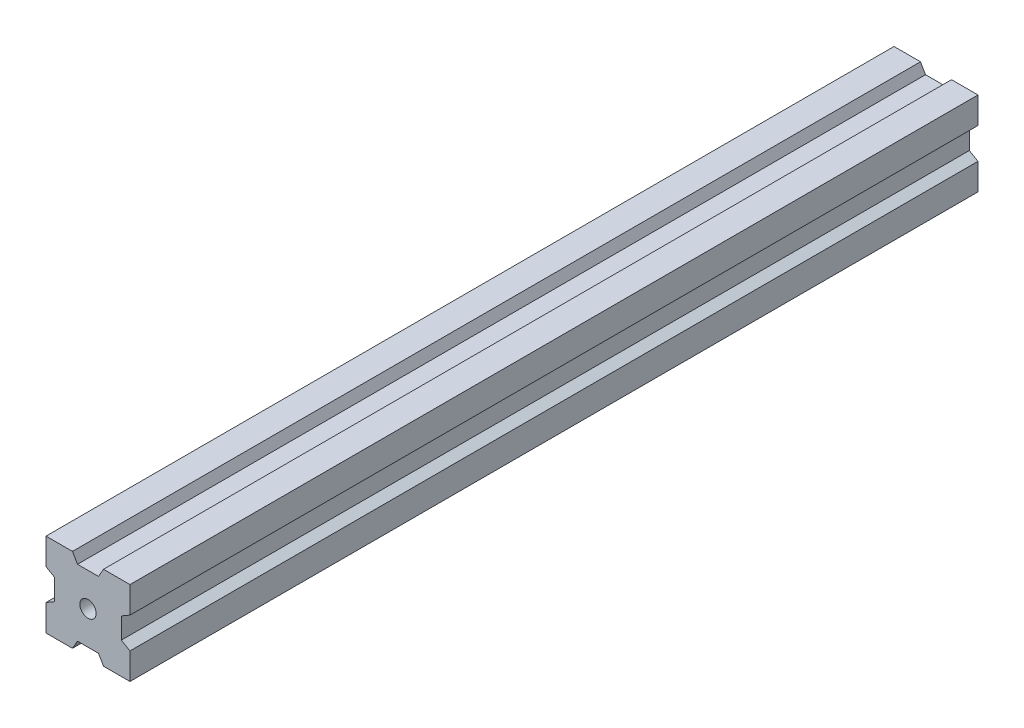
SolidWorks part; units mm, degrees
ref_plane "前视基准面" through (0, 0, 0) normal (0, 0, 1) x (1, 0, 0)
ref_plane "上视基准面" through (0, 0, 0) normal (0, 1, 0) x (1, 0, 0)
ref_plane "右视基准面" through (0, 0, 0) normal (1, 0, 0) x (0, 0, -1)
sketch "草图1" plane through (0, 0, 0) normal (0, 0, 1) x (1, 0, 0)
  line L1 (10, -10) -> (-10, -10)
  line L2 (10, -10) -> (10, 10)
  line L3 (10, 10) -> (-10, 10)
  line L4 (-10, -10) -> (-10, 10)
  line L5 (10, -10) -> (-10, 10) construction
  line L6 (10, 10) -> (-10, -10) construction
  circle A0 centre (0, 0) radius 1.9444
  point P0 (0, 0)
  dimension "D1" = 20
extrude "凸台-拉伸1" add sketch "草图1" along normal mid plane 202
sketch "草图2" plane through (0, 0, 101) normal (0, 0, 1) x (1, 0, 0)
  line L0 (-3.6944, 10) -> (-2.5, 7.9312)
  line L1 (10, 10) -> (-10, 10) construction
  line L2 (-2.5, 7.9312) -> (2.5, 7.9312)
  line L3 (2.5, 7.9312) -> (3.6944, 10)
  line L4 (0, 10) -> (0, 7.9312) construction
  line L5 (-3.6944, 10) -> (3.6944, 10) construction
  dimension "D1" = 5
  dimension "D2" = 60
extrude "切除-拉伸1" cut sketch "草图2" against normal through all and the other way through all
pattern_circular "阵列(圆周)1" count 4 over 360 about axis through (0, 0, 101) along (0, 0, -1) of "切除-拉伸1"
